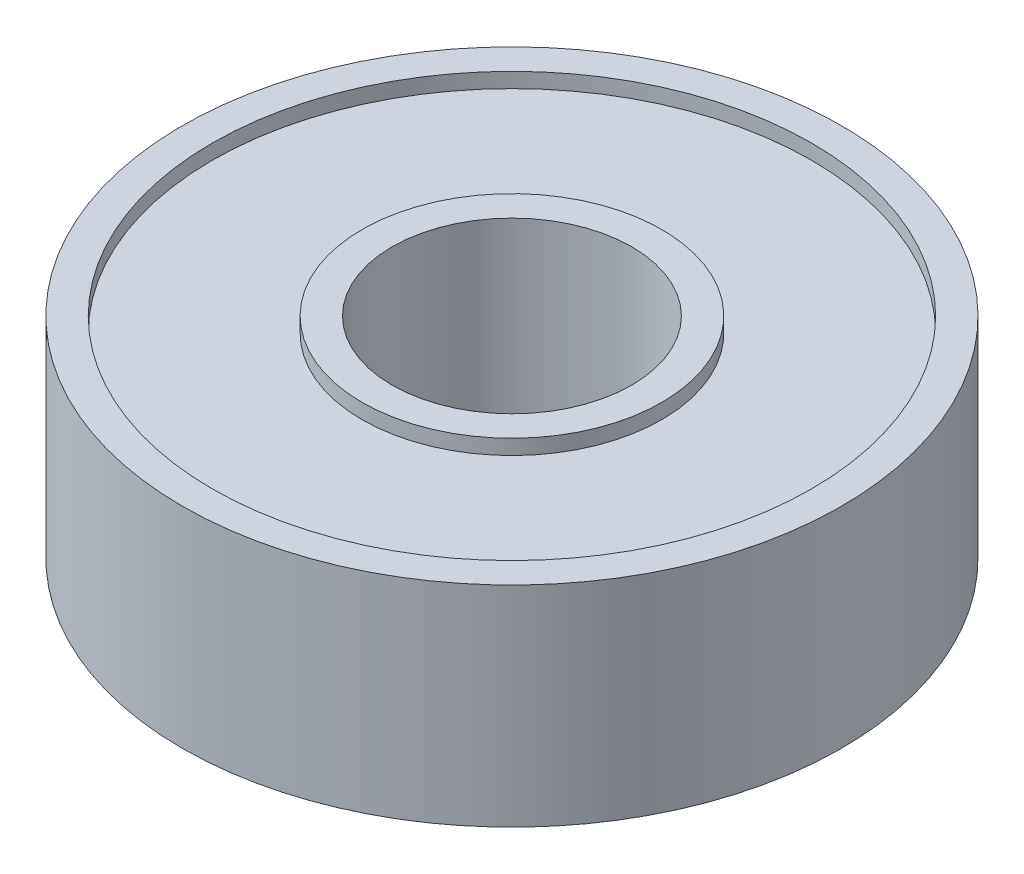
SolidWorks part; units mm, degrees
ref_plane "Front Plane" through (0, 0, 0) normal (0, 0, 1) x (1, 0, 0)
ref_plane "Top Plane" through (0, 0, 0) normal (0, 1, 0) x (1, 0, 0)
ref_plane "Right Plane" through (0, 0, 0) normal (1, 0, 0) x (0, 0, -1)
sketch "Sketch1" plane through (0, 0, 0) normal (0, 1, 0) x (1, 0, 0)
  circle A0 centre (0, 0) radius 11
  circle A1 centre (0, 0) radius 4
  dimension "D1" = 22
  dimension "D2" = 8
extrude "Boss-Extrude1" add sketch "Sketch1" along normal blind 7
sketch "Sketch2" plane through (0, 0, 0) normal (0, -1, 0) x (1, 0, 0)
  circle A0 centre (0, 0) radius 10
  circle A1 centre (0, 0) radius 11 construction
  circle A2 centre (0, 0) radius 5
  circle A3 centre (0, 0) radius 4 construction
  dimension "D1" = 1
  dimension "D2" = 1
extrude "Cut-Extrude1" cut sketch "Sketch2" against normal blind 0.5
sketch "Sketch3" plane through (0, 7, 0) normal (0, 1, 0) x (1, 0, 0)
  circle A0 centre (0, 0) radius 10
  circle A1 centre (0, 0) radius 5
  circle A2 centre (0, 0) radius 11 construction
  circle A3 centre (0, 0) radius 4 construction
  dimension "D1" = 1
  dimension "D2" = 1
extrude "Cut-Extrude2" cut sketch "Sketch3" against normal blind 0.5
